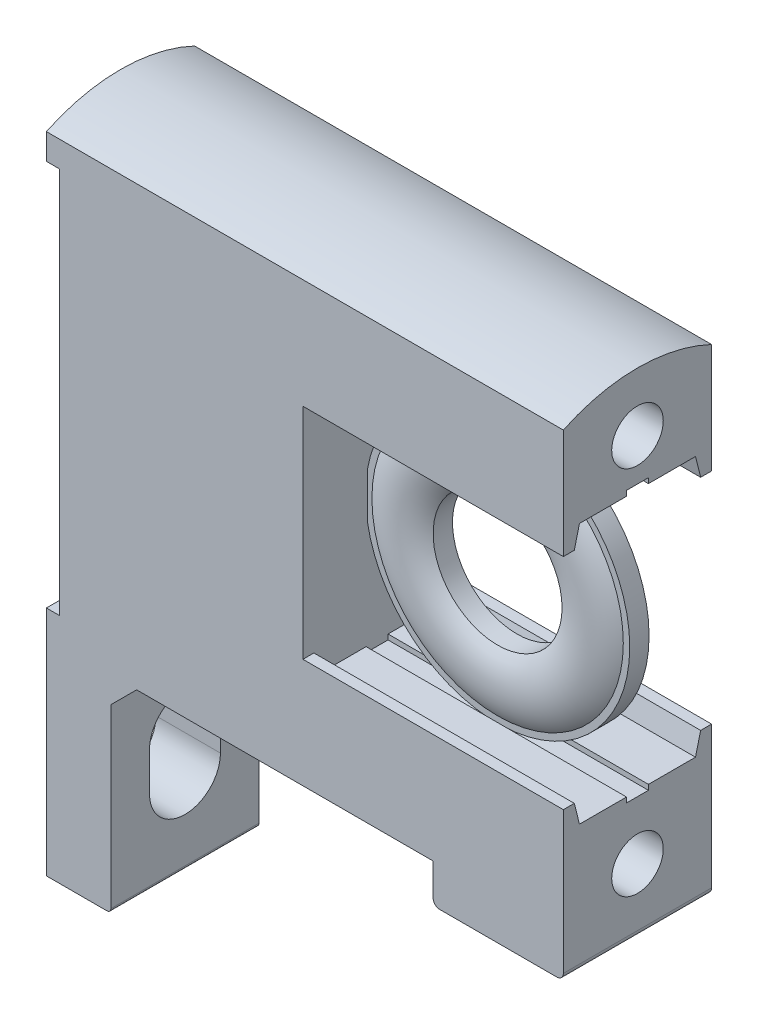
from build123d import *

# Parameters (mm, degrees)
EXTRUDE_1_DEPTH          = 5.75
EXTRUDE_1_DEPTH_BACK     = 5.75
CUT_EXTRUDE_1_DEPTH      = 30
EXTRUDE_2_DEPTH          = 40.1
CUT_EXTRUDE_2_DEPTH      = 20.2
CUT_EXTRUDE_3_DEPTH      = 4.25
CUT_EXTRUDE_3_DEPTH_BACK = 4.25
CUT_EXTRUDE_4_DEPTH      = 4.25
CUT_EXTRUDE_4_DEPTH_BACK = 4.25
CUT_EXTRUDE_5_DEPTH      = 4.25
CUT_EXTRUDE_5_DEPTH_BACK = 4.25
SKETCH_10_W              = 4
SKETCH_10_H              = 2


with BuildPart() as part:
    # 草图1 → 凸台-拉伸1 (new, two sides: drawn at the far end of the back side and taken through both)
    with BuildSketch(Plane.XY.offset(-EXTRUDE_1_DEPTH_BACK)):
        with BuildLine():
            Line((-30, 17), (-30, 15))
            Line((-30, 15), (-29, 15))
            Line((-29, 15), (-29, -15))
            Line((-29, -15), (-30, -15))
            Line((-30, -15), (-30, -33))
            Line((-30, -33), (-25.3, -33))
            ThreePointArc((-25.3, -33), (-25.087867966, -32.912132034), (-25, -32.7))
            Line((-25, -32.7), (-25, -19))
            Line((-25, -19), (-23, -17))
            Line((-23, -17), (0, -17))
            Line((0, -17), (0, -19.5))
            ThreePointArc((0, -19.5), (0.146446609, -19.853553391), (0.5, -20))
            Line((0.5, -20), (9.6, -20))
            ThreePointArc((9.6, -20), (9.953553391, -19.853553391), (10.1, -19.5))
            Line((10.1, -19.5), (10.1, 17))
            Line((10.1, 17), (-30, 17))
        make_face()
    extrude(amount=EXTRUDE_1_DEPTH + EXTRUDE_1_DEPTH_BACK)

    # 草图2 → 切除-拉伸1 (cut)
    with BuildSketch(Plane(origin=(0, 0, 0), x_dir=(0, 0, -1), z_dir=(1, 0, 0))):
        with BuildLine():
            Line((-2.75, -23.5), (-2.75, -26.5))
            ThreePointArc((-2.75, -26.5), (0, -29.25), (2.75, -26.5))
            Line((2.75, -26.5), (2.75, -23.5))
            ThreePointArc((2.75, -23.5), (0, -20.75), (-2.75, -23.5))
        make_face()
    extrude(amount=-CUT_EXTRUDE_1_DEPTH, mode=Mode.SUBTRACT)

    # 草图3 → 凸台-拉伸2 (add)
    with BuildSketch(Plane(origin=(10.1, 0, 0), x_dir=(0, 0, -1), z_dir=(1, 0, 0))):
        with BuildLine():
            Line((-5.75, 17), (5.75, 17))
            ThreePointArc((5.75, 17), (0, 18.299606469), (-5.75, 17))
        make_face()
    extrude(amount=-EXTRUDE_2_DEPTH)

    # 草图4 → 切除-旋转1 (revolve, cut)
    with BuildSketch(Plane.XY, mode=Mode.PRIVATE) as cut_revolve_1_sk:
        Polygon((4, -15), (4, -13), (11, -13), (11, -11.25), (14.5, -11.25), (15, -10.75), (15, -15), align=None)
    revolve(cut_revolve_1_sk.sketch.rotate(Axis((15, -15, 0), (-1, 0, 0)), 270), axis=Axis((15, -15, 0), (-1, 0, 0)), mode=Mode.SUBTRACT)

    # 草图5 → 切除-旋转2 (revolve, cut)
    with BuildSketch(Plane.XY, mode=Mode.PRIVATE) as cut_revolve_2_sk:
        Polygon((15, 13.75), (15, 9.5), (14.5, 10), (11, 10), (11, 11.75), (4, 11.75), (4, 13.75), align=None)
    revolve(cut_revolve_2_sk.sketch.rotate(Axis((4, 13.75, 0), (1, 0, 0)), 90), axis=Axis((4, 13.75, 0), (1, 0, 0)), mode=Mode.SUBTRACT)

    # 草图6 → 切除-拉伸2 (cut)
    with BuildSketch(Plane(origin=(10.1, 0, 0), x_dir=(0, 0, -1), z_dir=(1, 0, 0))):
        Polygon((-5.75, -8.5), (-4.9, -8.5), (-4.5, -10.1), (-0.85, -10.1), (-0.85, -10.5), (0.85, -10.5), (0.85, -10.1), (4.5, -10.1), (4.9, -8.5), (5.75, -8.5), (5.75, 8.5), (4.9, 8.5), (4.5, 10.1), (0.85, 10.1), (0.85, 10.5), (-0.85, 10.5), (-0.85, 10.1), (-4.5, 10.1), (-4.9, 8.5), (-5.75, 8.5), align=None)
    extrude(amount=-CUT_EXTRUDE_2_DEPTH, mode=Mode.SUBTRACT)

    # 草图7 → 旋转1 (revolve)
    with BuildSketch(Plane(origin=(0, 0, 0), x_dir=(0, 0, -1), z_dir=(1, 0, 0)), mode=Mode.PRIVATE) as revolve_1_sk:
        with BuildLine():
            Line((-0.75, 5), (0.75, 5))
            ThreePointArc((0.75, 5), (1.500003023, 7.375), (0.75, 9.75))
            Line((0.75, 9.75), (0.75, 10.25))
            Line((0.75, 10.25), (-0.75, 10.25))
            Line((-0.75, 10.25), (-0.75, 9.75))
            ThreePointArc((-0.75, 9.75), (-1.500003023, 7.375), (-0.75, 5))
        make_face()
    revolve(revolve_1_sk.sketch.rotate(Axis((0, 0, -50), (0, 0, 1)), 270), axis=Axis((0, 0, -50), (0, 0, 1)))

    # 草图8 → 切除-拉伸3 (cut, two sides: drawn at the far end of the back side and taken through both)
    with BuildSketch(Plane.XY.offset(-CUT_EXTRUDE_3_DEPTH_BACK)):
        Polygon((-29, 13.535533906), (-29, 1), (-13.535533906, 1), (-13.535533906, 8.535533906), (-8.535533906, 13.535533906), align=None)
    extrude(amount=CUT_EXTRUDE_3_DEPTH + CUT_EXTRUDE_3_DEPTH_BACK, mode=Mode.SUBTRACT)

    # 草图9 → 切除-拉伸4 (cut, two sides: drawn at the far end of the back side and taken through both)
    with BuildSketch(Plane.XY.offset(-CUT_EXTRUDE_4_DEPTH_BACK)):
        Polygon((-29, -13.535533906), (-8.535533906, -13.535533906), (-13.535533906, -8.535533906), (-13.535533906, -1), (-29, -1), align=None)
    extrude(amount=CUT_EXTRUDE_4_DEPTH + CUT_EXTRUDE_4_DEPTH_BACK, mode=Mode.SUBTRACT)

    # 草图10 → 切除-拉伸5 (cut, two sides: drawn at the far end of the back side and taken through both)
    with BuildSketch(Plane.XY.offset(-CUT_EXTRUDE_5_DEPTH_BACK)):
        with Locations((-27, 0)):
            Rectangle(SKETCH_10_W, SKETCH_10_H)
    extrude(amount=CUT_EXTRUDE_5_DEPTH + CUT_EXTRUDE_5_DEPTH_BACK, mode=Mode.SUBTRACT)


solid = part.part
